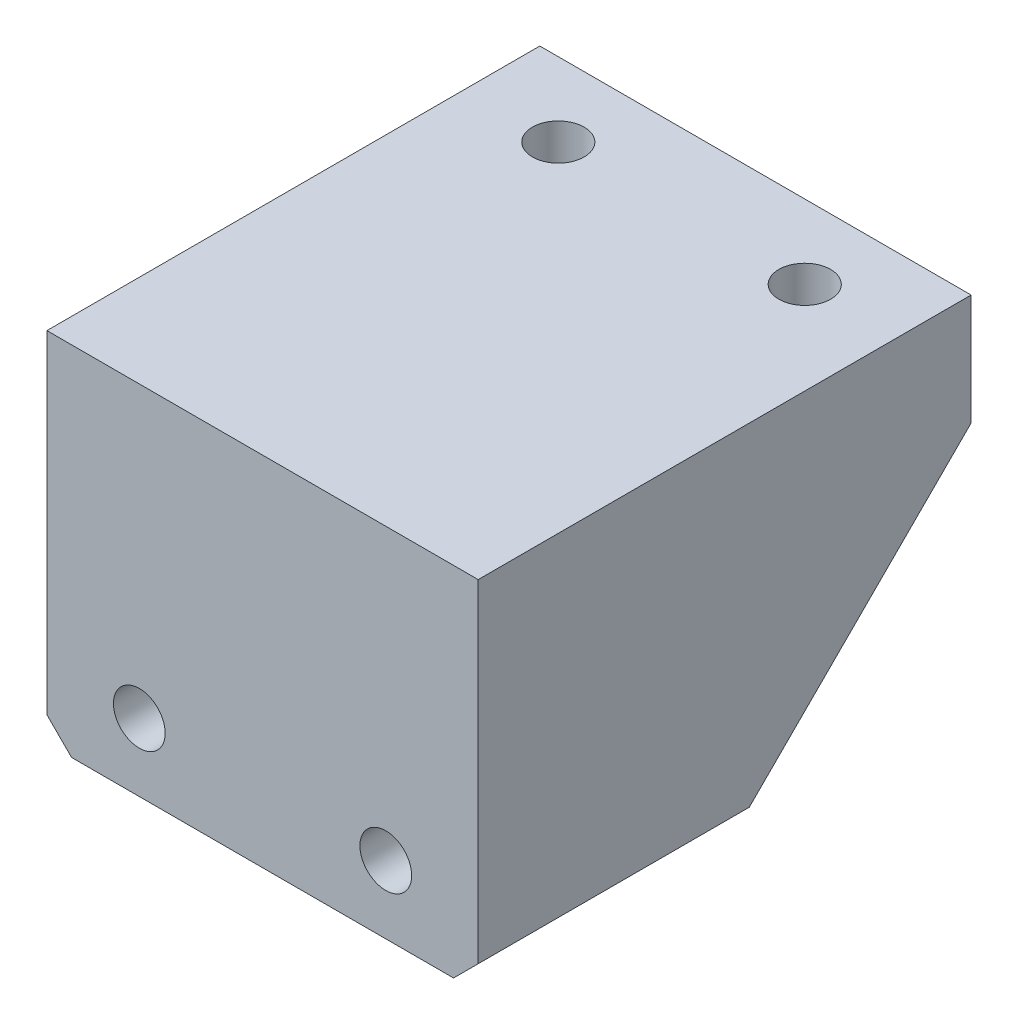
from build123d import *

# Parameters (mm, degrees)
SKETCH1_W             = 35
SKETCH1_H             = 40
BOSS_EXTRUDE1_DEPTH   = 29
CHAMFER1_SIZE         = 20
M5_TAPPED_HOLE1_D     = 4.2
M5_TAPPED_HOLE1_DEPTH = 12.4
M5_TAPPED_HOLE1_TIP   = 1.2618073
M5_TAPPED_HOLE2_D     = 4.2
CHAMFER2_SIZE         = 2


with BuildPart() as part:
    # Sketch1 → Boss-Extrude1 (new body)
    with BuildSketch(Plane(origin=(0, 0, 0), x_dir=(1, 0, 0), z_dir=(0, 1, 0))):
        Rectangle(SKETCH1_W, SKETCH1_H)
    extrude(amount=BOSS_EXTRUDE1_DEPTH)

    # Chamfer1
    chamfer1_edges = [part.edges().sort_by_distance(p)[0] for p in [
        (0, 0, -20),
    ]]
    chamfer(chamfer1_edges, length=CHAMFER1_SIZE)

    # M5 Tapped Hole1
    with Locations(Plane(origin=(-10, 5.5, 20), x_dir=(1, 0, 0), z_dir=(0, 0, 1))):
        with Locations((0, 0), (20, 0)):
            Hole(M5_TAPPED_HOLE1_D / 2, depth=M5_TAPPED_HOLE1_DEPTH)
            with Locations((0, 0, -(M5_TAPPED_HOLE1_DEPTH + M5_TAPPED_HOLE1_TIP / 2))):  # 118° drill point
                Cone(0, M5_TAPPED_HOLE1_D / 2, M5_TAPPED_HOLE1_TIP, mode=Mode.SUBTRACT)

    # M5 Tapped Hole2 (through all)
    with Locations(Plane(origin=(-10, 29, -14), x_dir=(0, 0, 1), z_dir=(0, 1, 0))):
        with Locations((0, 0), (0, 20)):
            Hole(M5_TAPPED_HOLE2_D / 2)

    # Chamfer2
    chamfer2_edges = [part.edges().sort_by_distance(p)[0] for p in [
        (-17.5, 0, 10),
        (17.5, 0, 10),
    ]]
    chamfer(chamfer2_edges, length=CHAMFER2_SIZE)


solid = part.part
